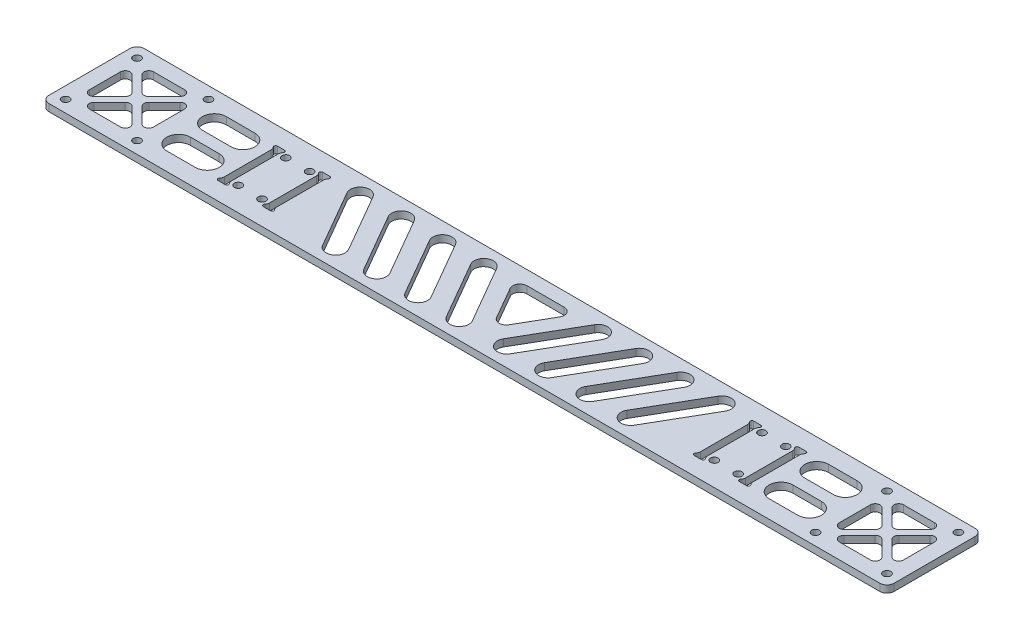
from build123d import *
from OCP.BRepFilletAPI import BRepFilletAPI_MakeFillet

# Parameters (mm, degrees)
SKETCH_1_R          = 1.6
SKETCH_1_W          = 3
SKETCH_1_H          = 25
EXTRUDE_1_DEPTH     = 3
SKETCH_2_R          = 0.75
CUT_EXTRUDE_1_DEPTH = 10
SKETCH_3_R          = 1.6
CUT_EXTRUDE_2_DEPTH = 179.648397698
CUT_EXTRUDE_3_DEPTH = 10
FILLET_1_R1         = 3
FILLET_1_R2         = 2


with BuildPart() as part:
    # 草图1 → 凸台-拉伸1 (new body)
    with BuildSketch(Plane(origin=(0, 0, 0), x_dir=(1, 0, 0), z_dir=(0, 1, 0))):
        with BuildLine():
            Line((-174.5, -20), (174.5, -20))
            ThreePointArc((174.5, -20), (176.621320344, -19.121320344), (177.5, -17))
            Line((177.5, -17), (177.5, 17))
            ThreePointArc((177.5, 17), (176.621320344, 19.121320344), (174.5, 20))
            Line((174.5, 20), (-174.5, 20))
            ThreePointArc((-174.5, 20), (-176.621320344, 19.121320344), (-177.5, 17))
            Line((-177.5, 17), (-177.5, -17))
            ThreePointArc((-177.5, -17), (-176.621320344, -19.121320344), (-174.5, -20))
        make_face()
        with Locations(Location((-172.5, 15, 0), (0, 0, 270))):
            Circle(SKETCH_1_R, mode=Mode.SUBTRACT)
        with Locations(Location((172.5, 15, 0), (0, 0, 90))):
            Circle(SKETCH_1_R, mode=Mode.SUBTRACT)
        with Locations(Location((-172.5, -15, 0), (0, 0, 270))):
            Circle(SKETCH_1_R, mode=Mode.SUBTRACT)
        with Locations(Location((172.5, -15, 0), (0, 0, 90))):
            Circle(SKETCH_1_R, mode=Mode.SUBTRACT)
        with Locations(Location((-142.5, 15, 0), (0, 0, 270))):
            Circle(SKETCH_1_R, mode=Mode.SUBTRACT)
        with Locations(Location((142.5, 15, 0), (0, 0, 90))):
            Circle(SKETCH_1_R, mode=Mode.SUBTRACT)
        with Locations(Location((-142.5, -15, 0), (0, 0, 270))):
            Circle(SKETCH_1_R, mode=Mode.SUBTRACT)
        with Locations(Location((142.5, -15, 0), (0, 0, 90))):
            Circle(SKETCH_1_R, mode=Mode.SUBTRACT)
        with Locations((109.5, 0)):
            Rectangle(SKETCH_1_W, SKETCH_1_H, mode=Mode.SUBTRACT)
        with Locations((-109.5, 0)):
            Rectangle(SKETCH_1_W, SKETCH_1_H, mode=Mode.SUBTRACT)
        with Locations((90.5, 0)):
            Rectangle(SKETCH_1_W, SKETCH_1_H, mode=Mode.SUBTRACT)
        with Locations((-90.5, 0)):
            Rectangle(SKETCH_1_W, SKETCH_1_H, mode=Mode.SUBTRACT)
    extrude(amount=EXTRUDE_1_DEPTH)

    # 草图2 → 切除-拉伸1 (cut)
    with BuildSketch(Plane(origin=(0, 3, 0), x_dir=(1, 0, 0), z_dir=(0, 1, 0))):
        with Locations((-111, 11.75)):
            Circle(SKETCH_2_R)
        with Locations((111, 11.75)):
            Circle(SKETCH_2_R)
        with Locations((-108, 11.75)):
            Circle(SKETCH_2_R)
        with Locations((108, 11.75)):
            Circle(SKETCH_2_R)
        with Locations((-92, 11.75)):
            Circle(SKETCH_2_R)
        with Locations((92, 11.75)):
            Circle(SKETCH_2_R)
        with Locations((-89, 11.75)):
            Circle(SKETCH_2_R)
        with Locations((89, 11.75)):
            Circle(SKETCH_2_R)
        with Locations((-89, -11.75)):
            Circle(SKETCH_2_R)
        with Locations((89, -11.75)):
            Circle(SKETCH_2_R)
        with Locations((-92, -11.75)):
            Circle(SKETCH_2_R)
        with Locations((92, -11.75)):
            Circle(SKETCH_2_R)
        with Locations((-108, -11.75)):
            Circle(SKETCH_2_R)
        with Locations((108, -11.75)):
            Circle(SKETCH_2_R)
        with Locations((-111, -11.75)):
            Circle(SKETCH_2_R)
        with Locations((111, -11.75)):
            Circle(SKETCH_2_R)
    extrude(amount=-CUT_EXTRUDE_1_DEPTH, mode=Mode.SUBTRACT)

    # 草图3 → 切除-拉伸2 (cut, through all)
    with BuildSketch(Plane(origin=(0, 3, 0), x_dir=(1, 0, 0), z_dir=(0, 1, 0))):
        with Locations(Location((-105, 10, 0), (0, 0, 270))):
            Circle(SKETCH_3_R)
        with Locations(Location((-105, -10, 0), (0, 0, 270))):
            Circle(SKETCH_3_R)
        with Locations(Location((-95, 10, 0), (0, 0, 270))):
            Circle(SKETCH_3_R)
        with Locations(Location((-95, -10, 0), (0, 0, 270))):
            Circle(SKETCH_3_R)
        with Locations(Location((95, -10, 0), (0, 0, 90))):
            Circle(SKETCH_3_R)
        with Locations(Location((95, 10, 0), (0, 0, 90))):
            Circle(SKETCH_3_R)
        with Locations(Location((105, -10, 0), (0, 0, 90))):
            Circle(SKETCH_3_R)
        with Locations(Location((105, 10, 0), (0, 0, 90))):
            Circle(SKETCH_3_R)
    extrude(amount=-CUT_EXTRUDE_2_DEPTH, mode=Mode.SUBTRACT)

    # 草图5 → 切除-拉伸3 (cut)
    with BuildSketch(Plane(origin=(0, 3, 0), x_dir=(1, 0, 0), z_dir=(0, 1, 0))):
        Polygon((-168.878679656, 13.5), (-157.5, 2.121320344), (-146.121320344, 13.5), align=None)
        Polygon((-171, -11.378679656), (-171, 11.378679656), (-159.621320344, 0), align=None)
        Polygon((-168.878679656, -13.5), (-146.121320344, -13.5), (-157.5, -2.121320344), align=None)
        Polygon((-144, -11.378679656), (-144, 11.378679656), (-155.378679656, 0), align=None)
        Polygon((171, -11.378679656), (159.621320344, 0), (171, 11.378679656), align=None)
        Polygon((168.878679656, -13.5), (157.5, -2.121320344), (146.121320344, -13.5), align=None)
        Polygon((155.378679656, 0), (144, -11.378679656), (144, 11.378679656), align=None)
        Polygon((157.5, 2.121320344), (146.121320344, 13.5), (168.878679656, 13.5), align=None)
        with BuildLine():
            Line((-132.5, 12.5), (-120.5, 12.5))
            ThreePointArc((-120.5, 12.5), (-115.5, 7.5), (-120.5, 2.5))
            Line((-120.5, 2.5), (-132.5, 2.5))
            ThreePointArc((-132.5, 2.5), (-137.5, 7.5), (-132.5, 12.5))
        make_face()
        with BuildLine():
            Line((132.5, 12.5), (120.5, 12.5))
            ThreePointArc((120.5, 12.5), (115.5, 7.5), (120.5, 2.5))
            Line((120.5, 2.5), (132.5, 2.5))
            ThreePointArc((132.5, 2.5), (137.5, 7.5), (132.5, 12.5))
        make_face()
        with BuildLine():
            Line((-132.5, -2.5), (-120.5, -2.5))
            ThreePointArc((-120.5, -2.5), (-115.5, -7.5), (-120.5, -12.5))
            Line((-120.5, -12.5), (-132.5, -12.5))
            ThreePointArc((-132.5, -12.5), (-137.5, -7.5), (-132.5, -2.5))
        make_face()
        with BuildLine():
            Line((132.5, -2.5), (120.5, -2.5))
            ThreePointArc((120.5, -2.5), (115.5, -7.5), (120.5, -12.5))
            Line((120.5, -12.5), (132.5, -12.5))
            ThreePointArc((132.5, -12.5), (137.5, -7.5), (132.5, -2.5))
        make_face()
        with BuildLine():
            Line((-72.497422612, 14.124355653), (-58.497422612, -10.124355653))
            ThreePointArc((-58.497422612, -10.124355653), (-59.961524227, -15.588457268), (-65.425625842, -14.124355653))
            Line((-65.425625842, -14.124355653), (-79.425625842, 10.124355653))
            ThreePointArc((-79.425625842, 10.124355653), (-77.961524227, 15.588457268), (-72.497422612, 14.124355653))
        make_face()
        with BuildLine():
            Line((72.497422612, 14.124355653), (58.497422612, -10.124355653))
            ThreePointArc((58.497422612, -10.124355653), (59.961524227, -15.588457268), (65.425625842, -14.124355653))
            Line((65.425625842, -14.124355653), (79.425625842, 10.124355653))
            ThreePointArc((79.425625842, 10.124355653), (77.961524227, 15.588457268), (72.497422612, 14.124355653))
        make_face()
        with BuildLine():
            Line((-55.176914536, 14.124355653), (-41.176914536, -10.124355653))
            ThreePointArc((-41.176914536, -10.124355653), (-42.641016151, -15.588457268), (-48.105117767, -14.124355653))
            Line((-48.105117767, -14.124355653), (-62.105117767, 10.124355653))
            ThreePointArc((-62.105117767, 10.124355653), (-60.641016151, 15.588457268), (-55.176914536, 14.124355653))
        make_face()
        with BuildLine():
            Line((55.176914536, 14.124355653), (41.176914536, -10.124355653))
            ThreePointArc((41.176914536, -10.124355653), (42.641016151, -15.588457268), (48.105117767, -14.124355653))
            Line((48.105117767, -14.124355653), (62.105117767, 10.124355653))
            ThreePointArc((62.105117767, 10.124355653), (60.641016151, 15.588457268), (55.176914536, 14.124355653))
        make_face()
        with BuildLine():
            Line((-37.856406461, 14.124355653), (-23.856406461, -10.124355653))
            ThreePointArc((-23.856406461, -10.124355653), (-25.320508076, -15.588457268), (-30.784609691, -14.124355653))
            Line((-30.784609691, -14.124355653), (-44.784609691, 10.124355653))
            ThreePointArc((-44.784609691, 10.124355653), (-43.320508076, 15.588457268), (-37.856406461, 14.124355653))
        make_face()
        with BuildLine():
            Line((37.856406461, 14.124355653), (23.856406461, -10.124355653))
            ThreePointArc((23.856406461, -10.124355653), (25.320508076, -15.588457268), (30.784609691, -14.124355653))
            Line((30.784609691, -14.124355653), (44.784609691, 10.124355653))
            ThreePointArc((44.784609691, 10.124355653), (43.320508076, 15.588457268), (37.856406461, 14.124355653))
        make_face()
        with BuildLine():
            Line((-20.535898385, 14.124355653), (-6.535898385, -10.124355653))
            ThreePointArc((-6.535898385, -10.124355653), (-8, -15.588457268), (-13.464101615, -14.124355653))
            Line((-13.464101615, -14.124355653), (-27.464101615, 10.124355653))
            ThreePointArc((-27.464101615, 10.124355653), (-26, 15.588457268), (-20.535898385, 14.124355653))
        make_face()
        with BuildLine():
            Line((20.535898385, 14.124355653), (6.535898385, -10.124355653))
            ThreePointArc((6.535898385, -10.124355653), (8, -15.588457268), (13.464101615, -14.124355653))
            Line((13.464101615, -14.124355653), (27.464101615, 10.124355653))
            ThreePointArc((27.464101615, 10.124355653), (26, 15.588457268), (20.535898385, 14.124355653))
        make_face()
        Polygon((13, 14.124355653), (-13, 14.124355653), (0, -8.392304845), align=None)
    extrude(amount=-CUT_EXTRUDE_3_DEPTH, mode=Mode.SUBTRACT)

    # 圆角1: one fillet with a radius per group of edges: ONE call of the kernel's fillet builder (fillet() takes one radius for all edges)
    fillet_1_edges_1 = [part.edges().sort_by_distance(p)[0] for p in [
        (13, 1.5, -14.124355653),
        (0, 1.5, 8.392304845),
        (-13, 1.5, -14.124355653),
    ]]
    fillet_1_edges_2 = [part.edges().sort_by_distance(p)[0] for p in [
        (-146.121320344, 1.5, -13.5),
        (-168.878679656, 1.5, -13.5),
        (-146.121320344, 1.5, 13.5),
        (-157.5, 1.5, 2.121320344),
        (-168.878679656, 1.5, 13.5),
        (-157.5, 1.5, -2.121320344),
        (-171, 1.5, 11.378679656),
        (-159.621320344, 1.5, 0),
        (-171, 1.5, -11.378679656),
        (155.378679656, 1.5, 0),
        (144, 1.5, -11.378679656),
        (144, 1.5, 11.378679656),
        (157.5, 1.5, -2.121320344),
        (168.878679656, 1.5, -13.5),
        (146.121320344, 1.5, -13.5),
        (146.121320344, 1.5, 13.5),
        (168.878679656, 1.5, 13.5),
        (157.5, 1.5, 2.121320344),
        (-144, 1.5, -11.378679656),
        (-155.378679656, 1.5, 0),
        (-144, 1.5, 11.378679656),
        (171, 1.5, 11.378679656),
        (171, 1.5, -11.378679656),
        (159.621320344, 1.5, 0),
        (-89, 1.5, -11),
        (-92, 1.5, -11),
        (-92, 1.5, 11),
        (-89, 1.5, 11),
        (-108, 1.5, -11),
        (-111, 1.5, -11),
        (-111, 1.5, 11),
        (-108, 1.5, 11),
        (111, 1.5, -11),
        (108, 1.5, -11),
        (108, 1.5, 11),
        (111, 1.5, 11),
        (92, 1.5, -11),
        (89, 1.5, -11),
        (89, 1.5, 11),
        (92, 1.5, 11),
    ]]
    fillet_1 = BRepFilletAPI_MakeFillet(part.part.solid().wrapped)
    for e in fillet_1_edges_1:
        fillet_1.Add(FILLET_1_R1, e.wrapped)
    for e in fillet_1_edges_2:
        fillet_1.Add(FILLET_1_R2, e.wrapped)
    add(Compound.cast(fillet_1.Shape()), mode=Mode.REPLACE)


solid = part.part
